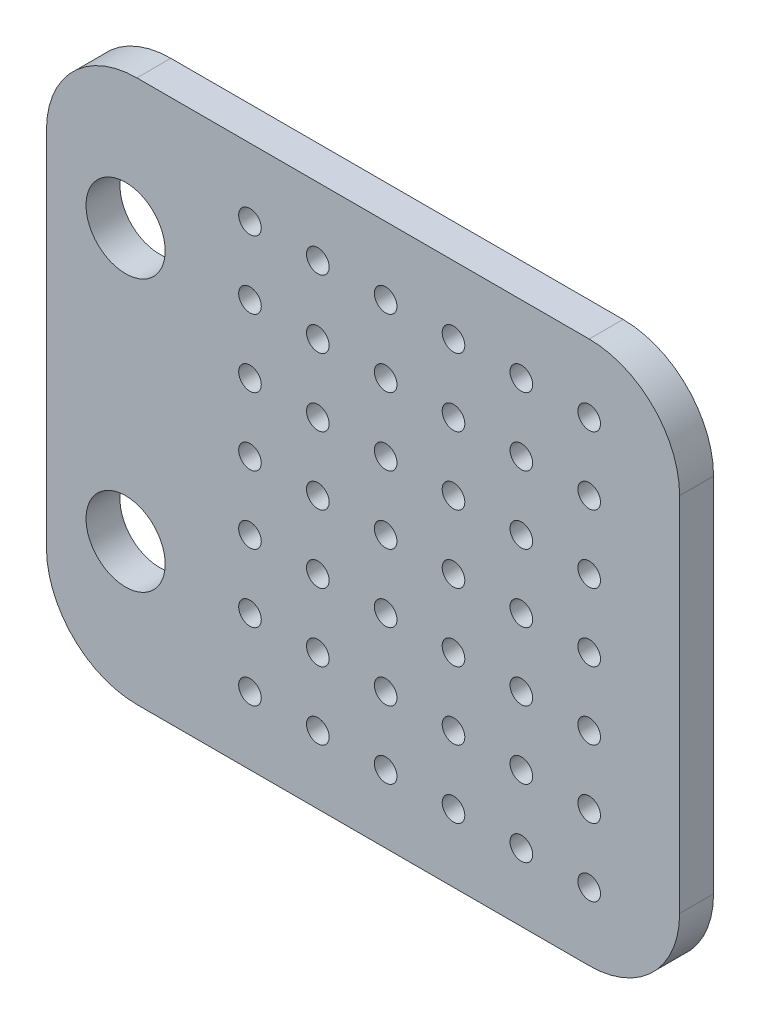
from build123d import *

# Parameters (mm, degrees)
SKETCH1_W                  = 28
SKETCH1_H                  = 24
BOSS_EXTRUDE1_DEPTH        = 0.75
FILLET1_R                  = 4
F_3_5_3_5_DIAMETER_HOLE1_D = 3.5
F_1_0_1_DIAMETER_HOLE1_D   = 1
LPATTERN1_COUNT            = 6
LPATTERN1_PITCH            = 3
LPATTERN1_COUNT_DIR2       = 7
LPATTERN1_PITCH_DIR2       = 3


with BuildPart() as part:
    # Sketch1 → Boss-Extrude1 (new, symmetric)
    with BuildSketch(Plane.XY):
        Rectangle(SKETCH1_W, SKETCH1_H)
    extrude(amount=BOSS_EXTRUDE1_DEPTH, both=True)

    # Fillet1
    fillet1_edges = [part.edges().sort_by_distance(p)[0] for p in [
        (14, -12, 0),
        (-14, -12, 0),
        (-14, 12, 0),
        (14, 12, 0),
    ]]
    fillet(fillet1_edges, radius=FILLET1_R)

    # Ø3.5 (3.5) Diameter Hole1 (through all)
    with Locations(Plane.XY.offset(0.75)):
        with Locations((-10.5, 6), (-10.5, -6)):
            Hole(F_3_5_3_5_DIAMETER_HOLE1_D / 2)

    # Ø1.0 (1) Diameter Hole1 (through all)
    with Locations(Plane.XY.offset(0.75)):
        with Locations((10, -9)):
            f_1_0_1_diameter_hole1 = Hole(F_1_0_1_DIAMETER_HOLE1_D / 2)

    # LPattern1: 1.0 _1_ Diameter Hole1 6 × 7
    with Locations(*[(-i * LPATTERN1_PITCH, j * LPATTERN1_PITCH_DIR2, 0) for i in range(LPATTERN1_COUNT) for j in range(LPATTERN1_COUNT_DIR2) if (i, j) != (0, 0)]):
        add(f_1_0_1_diameter_hole1, mode=Mode.SUBTRACT)


solid = part.part
